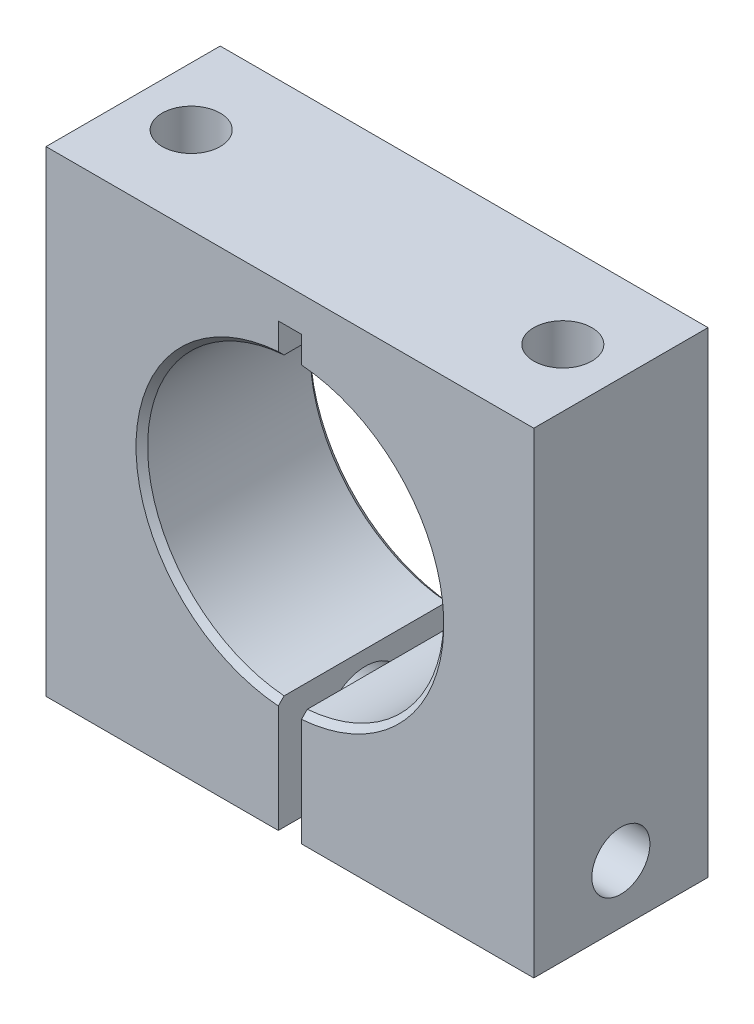
SolidWorks part; units mm, degrees
ref_plane "前视基准面" through (0, 0, 0) normal (0, 0, 1) x (1, 0, 0)
ref_plane "上视基准面" through (0, 0, 0) normal (0, 1, 0) x (1, 0, 0)
ref_plane "右视基准面" through (0, 0, 0) normal (1, 0, 0) x (0, 0, -1)
sketch "草图1" plane through (0, 0, 0) normal (0, 0, 1) x (1, 0, 0)
  line L1 (0, 0) -> (42, 0)
  line L2 (0, 0) -> (0, 41)
  line L3 (0, 41) -> (42, 41)
  line L4 (42, 0) -> (42, 41)
  dimension "D1" = 41
  dimension "D2" = 42
extrude "凸台-拉伸1" add sketch "草图1" along normal blind 15
sketch "草图2" plane through (0, 0, 15) normal (0, 0, 1) x (1, 0, 0)
  line L0 (21, 41) -> (21, 0) construction
  line L1 (42, 41) -> (0, 41) construction
  line L2 (0, 0) -> (42, 0) construction
  circle A0 centre (21, 22.5) radius 12.75
  dimension "D1" = 25.5
  dimension "D2" = 18.5
extrude "切除-拉伸1" cut sketch "草图2" against normal blind 15
sketch "草图3" plane through (0, 0, 15) normal (0, 0, 1) x (1, 0, 0)
  line L0 (0, 0) -> (42, 0) construction
  line L1 (20, 0) -> (22, 0)
  line L2 (20, 0) -> (20, 38)
  line L3 (20, 38) -> (22, 38)
  line L4 (22, 0) -> (22, 38)
  line L5 (21, 41) -> (21, -13.4566) construction
  line L6 (42, 41) -> (0, 41) construction
  dimension "D1" = 2
  dimension "D2" = 38
extrude "切除-拉伸2" cut sketch "草图3" against normal blind 15
hole_wizard "M6 螺纹孔1" positions "草图5" profile "草图4" tap size "M6" standard "ISO"
sketch "草图5" plane through (0, 41, 0) normal (0, 1, 0) x (1, 0, 0)
  line L0 (0, -7.5) -> (42, -7.5) construction
  line L1 (0, -15) -> (0, 0) construction
  line L2 (42, -15) -> (42, 0) construction
  line L4 (21, 0) -> (21, -15) construction
  line L5 (42, 0) -> (0, 0) construction
  line L6 (42, -15) -> (0, -15) construction
  point P0 (5, -7.5)
  point P2 (37, -7.5)
  dimension "D1" = 32
sketch "草图4" plane through (5, 41, 7.5) normal (1, 0, 0) x (0, 0, 1)
  line L0 (0, 0) -> (0, 18.5022)
  line L1 (0, 18.5022) -> (2.5, 17)
  line L2 (2.5, 17) -> (2.5, 0)
  line L5 (2.5, 0) -> (0, 0)
  line L10 (0, 18.5022) -> (-2.5, 17) construction
  line L11 (0, -6.35) -> (0, 107.95) construction
  dimension "螺纹孔钻头直径" = 5
  dimension "螺纹孔钻头深度" = 17
  dimension "导头角度" = 118
cosmetic thread "孔螺蚊线2" parameters "D1"=12, "D2"=6
cosmetic thread "孔螺蚊线4" parameters "D1"=12, "D2"=6
hole_wizard "Ø7.0 (7) 直径孔1" positions "草图7" profile "草图8" hole size "Ø7.0" standard "GB"
sketch "草图7" plane through (0, 0, 0) normal (-1, 0, 0) x (0, 0, 1)
  line L0 (15, 0) -> (0, 0) construction
  line L1 (7.5, 0) -> (7.5, 16.2376) construction
  point P0 (7.5, 5)
  dimension "D1" = 5
sketch "草图8" plane through (0, 5, 7.5) normal (0, 1, 0) x (0, 0, 1)
  line L0 (0, 0) -> (0, 20)
  line L1 (0, 20) -> (3.5, 20)
  line L2 (3.5, 20) -> (3.5, 0)
  line L5 (3.5, 0) -> (0, 0)
  line L11 (0, -6.35) -> (0, 107.95) construction
  dimension "通孔孔直径" = 7
  dimension "通孔孔深度" = 20
hole_wizard "M6 螺纹孔2" positions "草图10" profile "草图9" tap size "M6" standard "ISO" end condition up to next
sketch "草图10" plane through (22, 0, 0) normal (-1, 0, 0) x (0, 0, 1)
  point P0 (7.5, 5)
sketch "草图9" plane through (22, 5, 7.5) normal (0, 1, 0) x (0, 0, 1)
  line L0 (0, 0) -> (0, 20)
  line L1 (0, 20) -> (2.5, 20)
  line L2 (2.5, 20) -> (2.5, 0)
  line L5 (2.5, 0) -> (0, 0)
  line L11 (0, -6.35) -> (0, 107.95) construction
  dimension "通孔螺纹孔钻头直径" = 5
  dimension "通孔螺纹孔钻头深度" = 20
cosmetic thread "孔螺蚊线3" parameters "D2"=6
chamfer "倒角1" distance 0.5 angle 45 2 edges at (33.75, 22.5, 0) (33.75, 22.5, 15)
chamfer "倒角2" distance 0.5 angle 45 2 edges at (8.25, 22.5, 15) (8.25, 22.5, 0)
